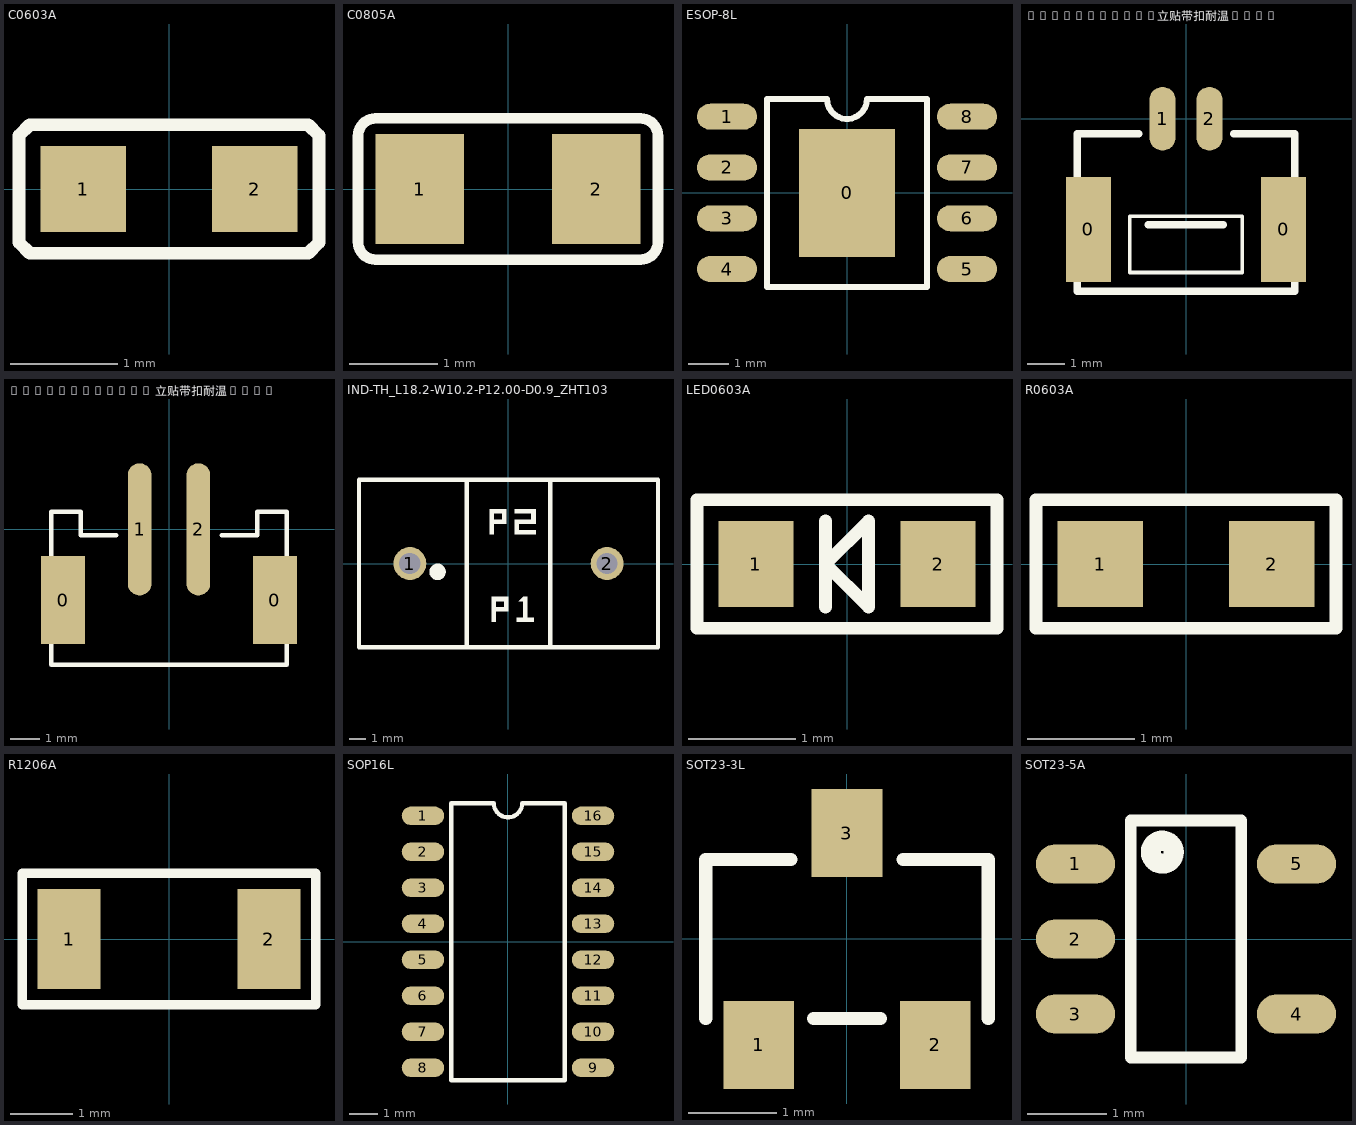
[diagram p0: the footprints below, top view; thin cyan lines are the x and y axes]
# Altium footprint library MISC75737-2.PcbLib: 12 footprints
Each footprint in its own frame and in the unit in brackets; x right, y up, seen from the top. Pads: shape width x height; smd on the part's side, far side on the other; paste and mask are expansions set on the pad; w line width, h text height; cw(c..) or ccw(c..) is an arc to the next point about the centre after c.

## C0603A [mm] "SMD capacitor"
pads (2):
  rect 0.8x0.8 smd mask+0.08: 1(-0.8,0) 2(0.8,0)
Top Overlay:
  lines w0.12: 0.551,-0.6 1.2,-0.6 ; -1.4,-0.5 -1.3,-0.6 1.3,-0.6 1.4,-0.5 1.4,0.5 1.3,0.6 -1.3,0.6 -1.4,0.5 -1.4,-0.5

## C0805A [mm] "SMD capacitor"
pads (2):
  rect 1x1.25 smd: 1(-1,0)
  rect 1x1.25 smd mask+0.102: 2(1,0)
Top Overlay:
  lines w0.12: -1.7,-0.6 ccw(c-1.5,-0.6) -1.5,-0.8 1.5,-0.8 ccw(c1.5,-0.6) 1.7,-0.6 1.7,0.6 ccw(c1.5,0.6) 1.5,0.8 -1.5,0.8 ccw(c-1.5,0.6) -1.7,0.6 -1.7,-0.6

## ESOP-8L [mm] "SMD MOS/IC"
pads (9):
  rect 2.4x3.2 smd: 0(0,0)
  oval 1.5x0.65 smd: 1(-3,1.905) 2(-3,0.635) 3(-3,-0.635) 4(-3,-1.905) 5(3,-1.905) 6(3,-0.635) 7(3,0.635) 8(3,1.905)
Top Overlay:
  lines w0.15: -2,-2.35 -2,2.35 -0.5,2.35 ccw(c0,2.35) 0.5,2.35 2,2.35 2,-2.35 -2,-2.35

## GH1.25-2PIN立贴带扣耐温260℃ [mm] "Vertical SMD with latch, rated 260℃"
pads (4):
  rect 1.2x2.8 smd: 0(-2.6,-2.95) 0(2.6,-2.95)
  oval 0.7x1.7 smd: 1(-0.625,0) 2(0.625,0)
Top Overlay:
  lines w0.1: -1.5,-4.1 -1.5,-2.6 1.5,-2.6 1.5,-4.1 -1.5,-4.1
  lines w0.2: -2.9,-0.4 -2.9,-4.6 2.9,-4.6 2.9,-0.4 1.27,-0.4 ; -2.895,-0.4 -1.265,-0.4 ; -1,-2.825 1,-2.825

## HY2.0WT-2A/P 立贴带扣耐温260℃ [mm] "Horizontal SMD connector"
pads (4):
  rect 1.5x3 smd: 0(-3.6,-2.4) 0(3.6,-2.4)
  oval 0.8x4.5 smd: 1(-1,0) 2(1,0)
Top Overlay:
  lines w0.15: -1.8,-0.2 -3,-0.2 -3,0.6 -4,0.6 -4,-4.6 4,-4.6 4,0.6 3,0.6 3,-0.2 1.8,-0.2

## IND-TH_L18.2-W10.2-P12.00-D0.9_ZHT103 [mm]
pads (2):
  round 2 hole 1.3: 1(-6,0) 2(6,0)
Top Overlay:
  circle w0.5: c-4.318,-0.508 r0.25
  region: 0.635,-2.286 0.889,-2.032 1.143,-2.032 1.143,-3.302 1.524,-3.302 1.524,-3.556 0.508,-3.556 0.508,-3.302 0.889,-3.302 0.889,-2.286
  region: -0.762,-2.032 0,-2.032 0,-2.921 -0.762,-2.921 -0.762,-2.667 -0.254,-2.667 -0.254,-2.286 -0.762,-2.286
  region: -1.016,-2.032 -1.016,-3.556 -0.762,-3.556 -0.762,-2.032
  region: -0.889,3.302 -0.127,3.302 -0.127,2.413 -0.889,2.413 -0.889,2.667 -0.381,2.667 -0.381,3.048 -0.889,3.048
  region: -1.143,3.302 -1.143,1.778 -0.889,1.778 -0.889,3.302
  region: 0.381,3.302 1.651,3.302 1.651,3.048 1.651,2.413 0.635,2.413 0.635,2.032 1.651,2.032 1.651,1.778 0.381,1.778 0.381,2.667 1.397,2.667 1.397,3.048 0.381,3.048
  lines w0.254: -9.1,-5.1 9.1,-5.1 9.1,5.1 -9.1,5.1 -9.1,-5.1 ; -2.54,-5.08 2.54,-5.08 2.54,5.08 -2.54,5.08 -2.54,-5.08
Mechanical 8:
  region: -9.04,-5.1 -9.04,-5.125 -9.075,-5.16 -9.125,-5.16 -9.16,-5.125 -9.16,-5.1 -9.16,-5.075 -9.125,-5.04 -9.075,-5.04 -9.04,-5.075 -9.04,-5.1

## LED0603A [mm] "SMD LED"
pads (2):
  rect 0.7x0.8 smd: 1(-0.85,0) 2(0.85,0)
Top Overlay:
  lines w0.12: -0.2,-0.4 -0.2,0.4 ; -1.4,-0.6 1.4,-0.6 1.4,0.6 -1.4,0.6 -1.4,-0.6 ; -0.2,0 0.2,-0.4 0.2,0.4 -0.2,0

## R0603A [mm] "SMD resistor"
height 0.5
pads (2):
  rect 0.8x0.8 smd mask+0.08: 1(-0.8,0) 2(0.8,0)
Top Overlay:
  lines w0.12: -1.4,-0.6 1.4,-0.6 1.4,0.6 -1.4,0.6 -1.4,-0.6

## R1206A [mm] "SMD resistor"
pads (2):
  rect 1x1.6 smd: 1(-1.6,0) 2(1.6,0)
Top Overlay:
  lines w0.15: -2.35,-1.05 -2.35,1.05 2.35,1.05 2.35,-1.05 -2.35,-1.05

## SOP16L [mm]
pads (16):
  oval 1.5x0.65 smd: 1(-3,4.445) 2(-3,3.175) 3(-3,1.905) 4(-3,0.635) 5(-3,-0.635) 6(-3,-1.905) 7(-3,-3.175) 8(-3,-4.445) 9(3,-4.445) 10(3,-3.175) 11(3,-1.905) 12(3,-0.635) 13(3,0.635) 14(3,1.905) 15(3,3.175) 16(3,4.445)
Top Overlay:
  lines w0.15: -2,-4.89 -2,4.89 -0.5,4.89 ccw(c0,4.89) 0.5,4.89 2,4.89 2,-4.89 -2,-4.89

## SOT23-3L [mm] "SMD MOS"
pads (3):
  rect 0.8x1 smd: 1(-1,-1.2) 2(1,-1.2) 3(0,1.2)
Top Overlay:
  lines w0.15: -1.6,-0.9 -1.6,0.9 -0.635,0.9 ; -0.381,-0.9 0.381,-0.9 ; 0.635,0.9 1.6,0.9 1.6,-0.9

## SOT23-5A [mm] "SMD IC"
pads (5):
  oval 1x0.5 smd mask+0.05: 1(-1.4,0.95) 2(-1.4,0) 3(-1.4,-0.95) 4(1.4,-0.95) 5(1.4,0.95)
Top Overlay:
  circle w0.254: c-0.3,1.1 r0.146
  lines w0.15: -0.7,-1.5 -0.7,1.5 0.7,1.5 0.7,-1.5 -0.7,-1.5